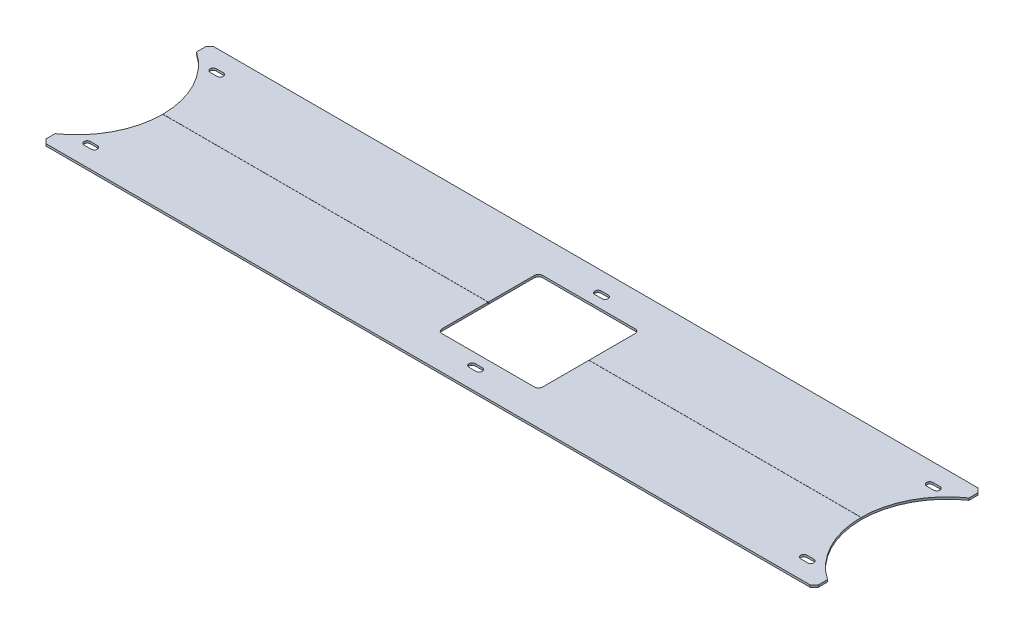
SolidWorks part; units mm, degrees
ref_plane "Front Plane" through (0, 0, 0) normal (0, 0, 1) x (1, 0, 0)
ref_plane "Top Plane" through (0, 0, 0) normal (0, 1, 0) x (1, 0, 0)
ref_plane "Right Plane" through (0, 0, 0) normal (1, 0, 0) x (0, 0, -1)
sketch "Sketch1" plane through (0, 0, 0) normal (0, 1, 0) x (1, 0, 0)
  line L1 (-276, 60) -> (276, 60)
  line L2 (-276, 60) -> (-276, -60)
  line L3 (-276, -60) -> (276, -60)
  line L4 (276, 60) -> (276, -60)
  line L5 (-276, 60) -> (276, -60) construction
  line L6 (-276, -60) -> (276, 60) construction
  point P0 (0, 0)
  dimension "D1" = 120
  dimension "D2" = 552
extrude "Boss-Extrude1" add sketch "Sketch1" along normal blind 1.5
chamfer "Chamfer1" distance 3 angle 45 2 edges at (276, 0.75, -60) (276, 0.75, 60)
chamfer "Chamfer2" distance 3 angle 45 2 edges at (-276, 0.75, -60) (-276, 0.75, 60)
sketch "Sketch12" plane through (0, 1.5, 0) normal (0, 1, 0) x (1, 0, 0)
  line L0 (-258.5, 45) -> (-253.5, 45) construction
  line L1 (-258.5, 47.25) -> (-253.5, 47.25)
  line L2 (-258.5, 42.75) -> (-253.5, 42.75)
  line L3 (-258.5, -45) -> (-253.5, -45) construction
  line L4 (-258.5, -42.75) -> (-253.5, -42.75)
  line L5 (-258.5, -47.25) -> (-253.5, -47.25)
  line L6 (0, 0) -> (-462.1641, 0) construction
  line L7 (-276, 57) -> (-276, -57) construction
  line L8 (273, 60) -> (-273, 60) construction
  arc A0 (-258.5, 47.25) -> (-258.5, 42.75) centre (-258.5, 45) ccw
  arc A1 (-253.5, 42.75) -> (-253.5, 47.25) centre (-253.5, 45) ccw
  arc A2 (-258.5, -42.75) -> (-258.5, -47.25) centre (-258.5, -45) ccw
  arc A3 (-253.5, -47.25) -> (-253.5, -42.75) centre (-253.5, -45) ccw
  point P2 (-256, 45)
  point P7 (-256, -45)
  dimension "D1" = 4.5
  dimension "D2" = 5
  dimension "D3" = 20
  dimension "D4" = 15
extrude "Cut-Extrude6" cut sketch "Sketch12" against normal through all
sketch "Sketch13" plane through (0, 1.5, 0) normal (0, 1, 0) x (1, 0, 0)
  line L0 (276, -57) -> (276, 57) construction
  line L1 (-276, 0.05) -> (276, 0.05)
  line L2 (-276, 0.05) -> (-276, -0.05)
  line L3 (-276, -0.05) -> (276, -0.05)
  line L4 (276, 0.05) -> (276, -0.05)
  line L5 (-276, 0.05) -> (276, -0.05) construction
  line L6 (-276, -0.05) -> (276, 0.05) construction
  line L7 (-276, 57) -> (-276, -57) construction
  point P0 (0, 0)
  dimension "D1" = 0.1
extrude "Cut-Extrude7" cut sketch "Sketch13" against normal through all
sketch "Sketch15" plane through (0, 1.5, 0) normal (0, 1, 0) x (1, 0, 0)
  line L0 (-276, -0.05) -> (276, -0.05) construction
  line L1 (52, 35.95) -> (-14, 35.95)
  line L2 (55, 32.95) -> (55, -33.05)
  line L3 (52, -36.05) -> (-14, -36.05)
  line L4 (-17, 32.95) -> (-17, -33.05)
  line L5 (55, 35.95) -> (-17, -36.05) construction
  line L6 (55, -36.05) -> (-17, 35.95) construction
  line L7 (-276, 57) -> (-276, 0.05) construction
  arc A0 (-17, -33.05) -> (-14, -36.05) centre (-14, -33.05) ccw
  arc A1 (55, -33.05) -> (52, -36.05) centre (52, -33.05) cw
  arc A2 (55, 32.95) -> (52, 35.95) centre (52, 32.95) ccw
  arc A3 (-14, 35.95) -> (-17, 32.95) centre (-14, 32.95) ccw
  point P0 (19, -0.05)
  dimension "D3" = 3
  dimension "D1" = 72
  dimension "D2" = 72
  dimension "D4" = 295
extrude "Cut-Extrude9" cut sketch "Sketch15" against normal through all
sketch "Sketch16" plane through (0, 1.5, 0) normal (0, 1, 0) x (1, 0, 0)
  line L0 (276, 0.05) -> (276, 57) construction
  line L1 (0, 0) -> (352.5911, 0) construction
  line L2 (0, 0) -> (0, 143.0362) construction
  circle A0 centre (311, 0) radius 61.5
  circle A1 centre (-311, 0) radius 61.5
  dimension "D1" = 123
  dimension "D2" = 35
extrude "Cut-Extrude10" cut sketch "Sketch16" against normal blind 10
mirror "Mirror1" about plane through (0, 0, 0) normal (1, 0, 0) of "Cut-Extrude6"
sketch "Sketch17" plane through (0, 0, 0) normal (0, -1, 0) x (1, 0, 0)
  line L0 (21.5, -45) -> (16.5, -45) construction
  line L1 (21.5, -47.25) -> (16.5, -47.25)
  line L2 (21.5, -42.75) -> (16.5, -42.75)
  line L3 (21.5, 45) -> (16.5, 45) construction
  line L4 (21.5, 42.75) -> (16.5, 42.75)
  line L5 (21.5, 47.25) -> (16.5, 47.25)
  line L6 (19, -35.95) -> (19, 67.0802) construction
  line L7 (52, -35.95) -> (-14, -35.95) construction
  line L8 (0, 0) -> (30.2672, 0) construction
  arc A0 (21.5, -47.25) -> (21.5, -42.75) centre (21.5, -45) ccw
  arc A1 (16.5, -42.75) -> (16.5, -47.25) centre (16.5, -45) ccw
  arc A2 (21.5, 42.75) -> (21.5, 47.25) centre (21.5, 45) ccw
  arc A3 (16.5, 47.25) -> (16.5, 42.75) centre (16.5, 45) ccw
  point P2 (19, -45)
  point P7 (19, 45)
  dimension "D1" = 5
  dimension "D2" = 4.5
  dimension "D3" = 90
extrude "Cut-Extrude11" cut sketch "Sketch17" against normal blind 10
